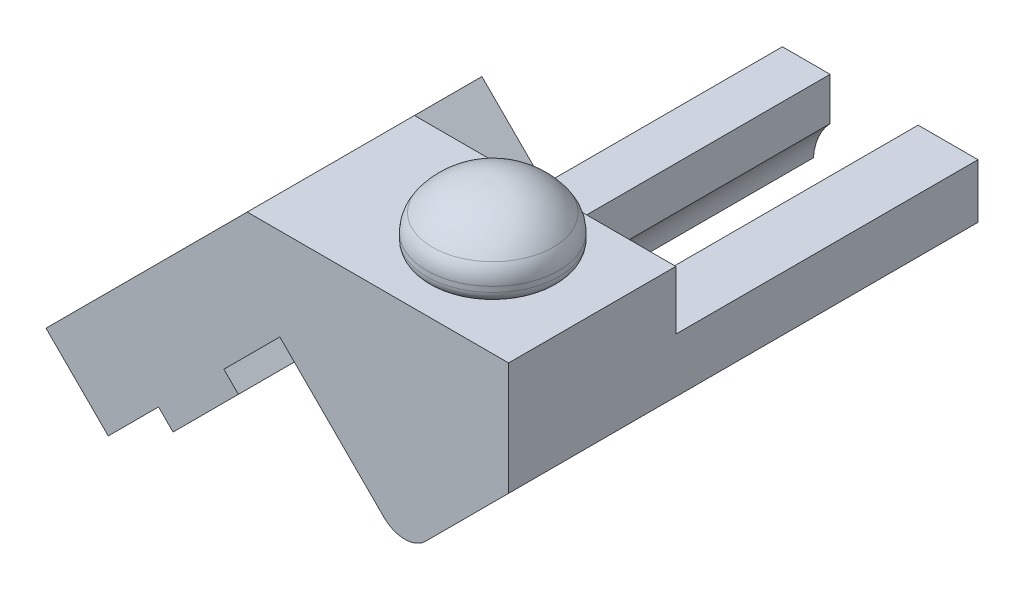
from build123d import *

# Parameters (mm, degrees)
BOSS_EXTRUDE1_DEPTH = 16
SKETCH2_W           = 8.91
SKETCH2_H           = 2
CUT_EXTRUDE1_DEPTH  = 10.3
CUT_EXTRUDE2_DEPTH  = 14.5
CUT_EXTRUDE3_DEPTH  = 14.5
BOSS_EXTRUDE2_DEPTH = 8


with BuildPart() as part:
    # Sketch1 → Boss-Extrude1 (new body)
    with BuildSketch(Plane.XY.offset(-14.5)):
        with BuildLine():
            Line((-5.37, 4.89), (-5.37, 0.647359313))
            Line((-5.37, 0.647359313), (-4.258679656, 1.758679656))
            Line((-4.258679656, 1.758679656), (-0.707106781, -1.792893219))
            ThreePointArc((-0.707106781, -1.792893219), (0, -2.085786438), (0.707106781, -1.792893219))
            Line((0.707106781, -1.792893219), (3.54, 1.04))
            Line((3.54, 1.04), (3.54, 4.89))
            Line((3.54, 4.89), (-5.37, 4.89))
        make_face()
    extrude(amount=BOSS_EXTRUDE1_DEPTH)

    # Sketch2 → Cut-Extrude1 (cut)
    with BuildSketch(Plane.XY.offset(-14.5)):
        with Locations((-0.915, 3.89)):
            Rectangle(SKETCH2_W, SKETCH2_H)
    extrude(amount=CUT_EXTRUDE1_DEPTH, mode=Mode.SUBTRACT)

    # Sketch3 → Cut-Extrude2 (cut)
    with BuildSketch(Plane.XY):
        with BuildLine():
            Line((-2.64, 0.14), (-2.64, -5))
            Line((-2.64, -5), (2.64, -5))
            Line((2.64, -5), (2.64, 0.14))
            Line((2.64, 0.14), (2.567267895, 0.067267895))
            ThreePointArc((2.567267895, 0.067267895), (2.355135861, -0.020600071), (2.143003826, 0.067267895))
            Line((2.143003826, 0.067267895), (2.070271721, 0.14))
            ThreePointArc((2.070271721, 0.14), (1.898724344, 0.836941375), (1.5, 1.433745096))
            Line((1.5, 1.433745096), (1.5, 2.89))
            Line((1.5, 2.89), (-1.5, 2.89))
            Line((-1.5, 2.89), (-1.5, 1.433745096))
            ThreePointArc((-1.5, 1.433745096), (-1.898724344, 0.836941375), (-2.070271721, 0.14))
            Line((-2.070271721, 0.14), (-2.143003826, 0.067267895))
            ThreePointArc((-2.143003826, 0.067267895), (-2.355135861, -0.020600071), (-2.567267895, 0.067267895))
            Line((-2.567267895, 0.067267895), (-2.64, 0.14))
        make_face()
    extrude(amount=-CUT_EXTRUDE2_DEPTH, mode=Mode.SUBTRACT)

    # Sketch4 → Cut-Extrude3 (cut)
    with BuildSketch(Plane.XY):
        Polygon((-5.37, 0.647359313), (-3.127359313, 2.89), (-5.37, 2.89), align=None)
    extrude(amount=-CUT_EXTRUDE3_DEPTH, mode=Mode.SUBTRACT)

    # Sketch5 → Boss-Extrude2 (add)
    with BuildSketch(Plane.XY.offset(-6.5)):
        Polygon((-12.228935778, -1.968935778), (-10.107615434, -4.090256121), (-8.39288149, -2.375522177), (-7.897906743, -2.870496924), (-5.670520382, -0.643110563), (-6.165495129, -0.148135816), (-3.248679656, 2.768679656), (-5.37, 4.89), align=None)
    extrude(amount=BOSS_EXTRUDE2_DEPTH)

    # Sketch6 → Cut-Revolve1 (revolve, cut)
    with BuildSketch(Plane.XY.offset(-2.5), mode=Mode.PRIVATE) as cut_revolve1_sk:
        Polygon((-5.894974747, -2.676042559), (-6.955634919, -3.73670273), (-10.491168825, -0.201168825), (-9.430508653, 0.859491347), align=None)
    revolve(cut_revolve1_sk.sketch.rotate(Axis((-9.430508653, 0.859491347, -2.5), (0.7071067811865479, -0.7071067811865472, 0)), 180), axis=Axis((-9.430508653, 0.859491347, -2.5), (0.7071067811865479, -0.7071067811865472, 0)), mode=Mode.SUBTRACT)

    # Sketch7 → Revolve1 (revolve)
    with BuildSketch(Plane(origin=(0, 0, 0), x_dir=(0, 0, -1), z_dir=(1, 0, 0)), mode=Mode.PRIVATE) as revolve1_sk:
        with BuildLine():
            Line((1.5, 4.69), (-0.7, 4.69))
            Line((-0.7, 4.69), (-0.7, 4.89))
            Line((-0.7, 4.89), (-0.35, 4.89))
            ThreePointArc((-0.35, 4.89), (-0.632842712, 5.007157288), (-0.75, 5.29))
            Line((-0.75, 5.29), (-0.75, 5.470108292))
            ThreePointArc((-0.75, 5.470108292), (-0.700420617, 5.781075575), (-0.556598698, 6.061207725))
            ThreePointArc((-0.556598698, 6.061207725), (0.348255742, 6.809981308), (1.5, 7.04))
            Line((1.5, 7.04), (1.5, 4.69))
        make_face()
    revolve(revolve1_sk.sketch.rotate(Axis((0, 7.04, -1.5), (0, -1, 0)), 180), axis=Axis((0, 7.04, -1.5), (0, -1, 0)))


solid = part.part
